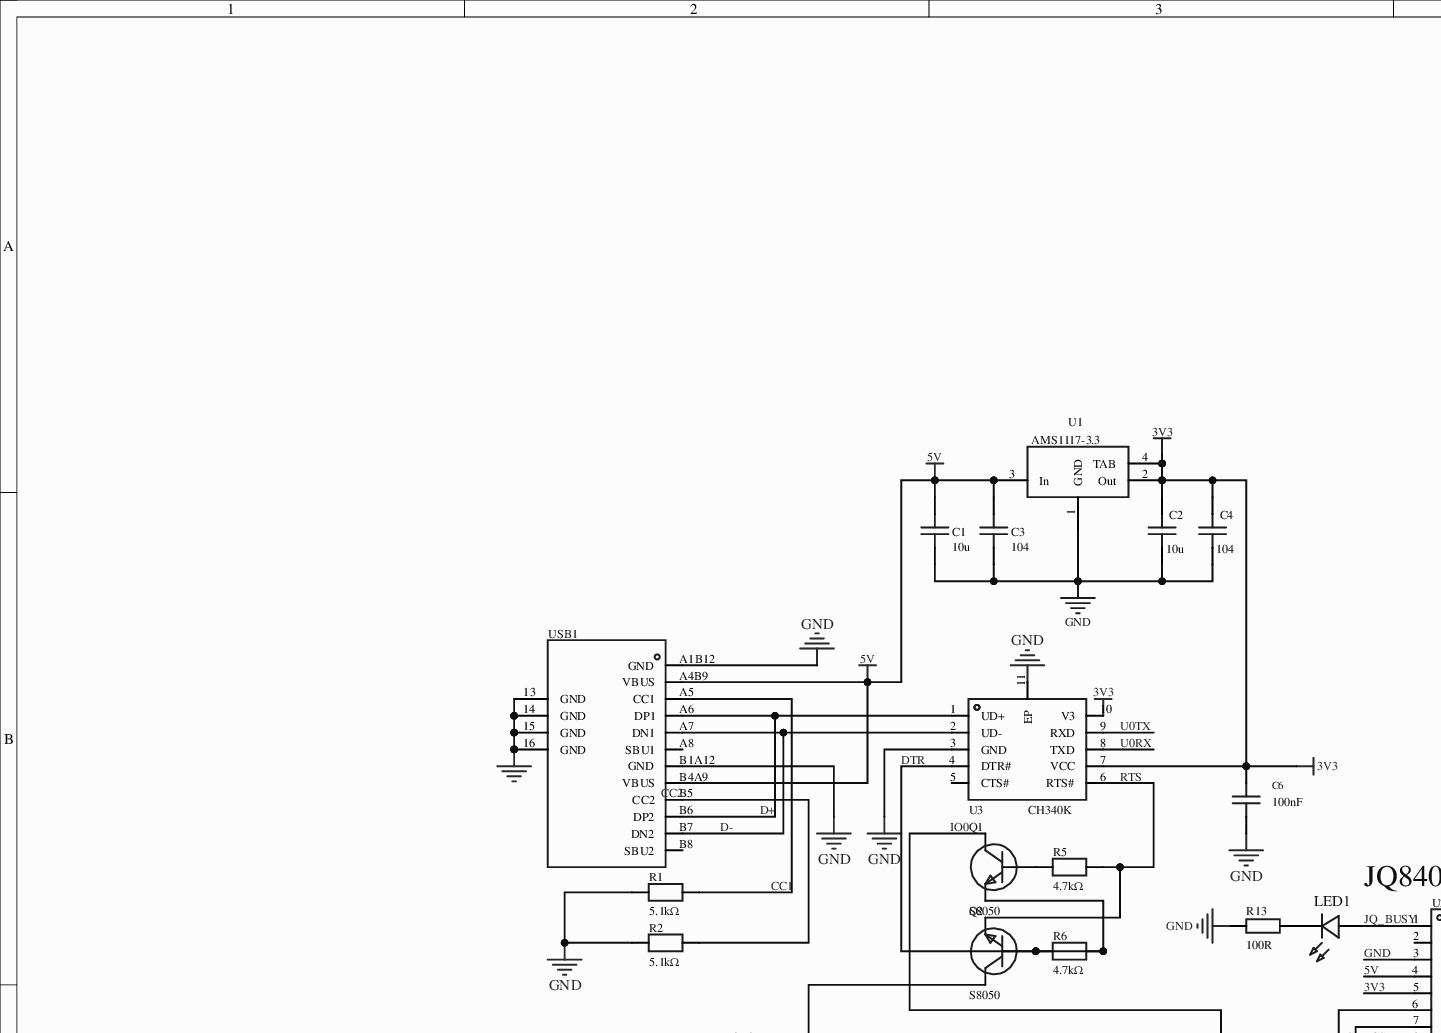
[diagram p0: MISC50923-3.schdoc, top left]
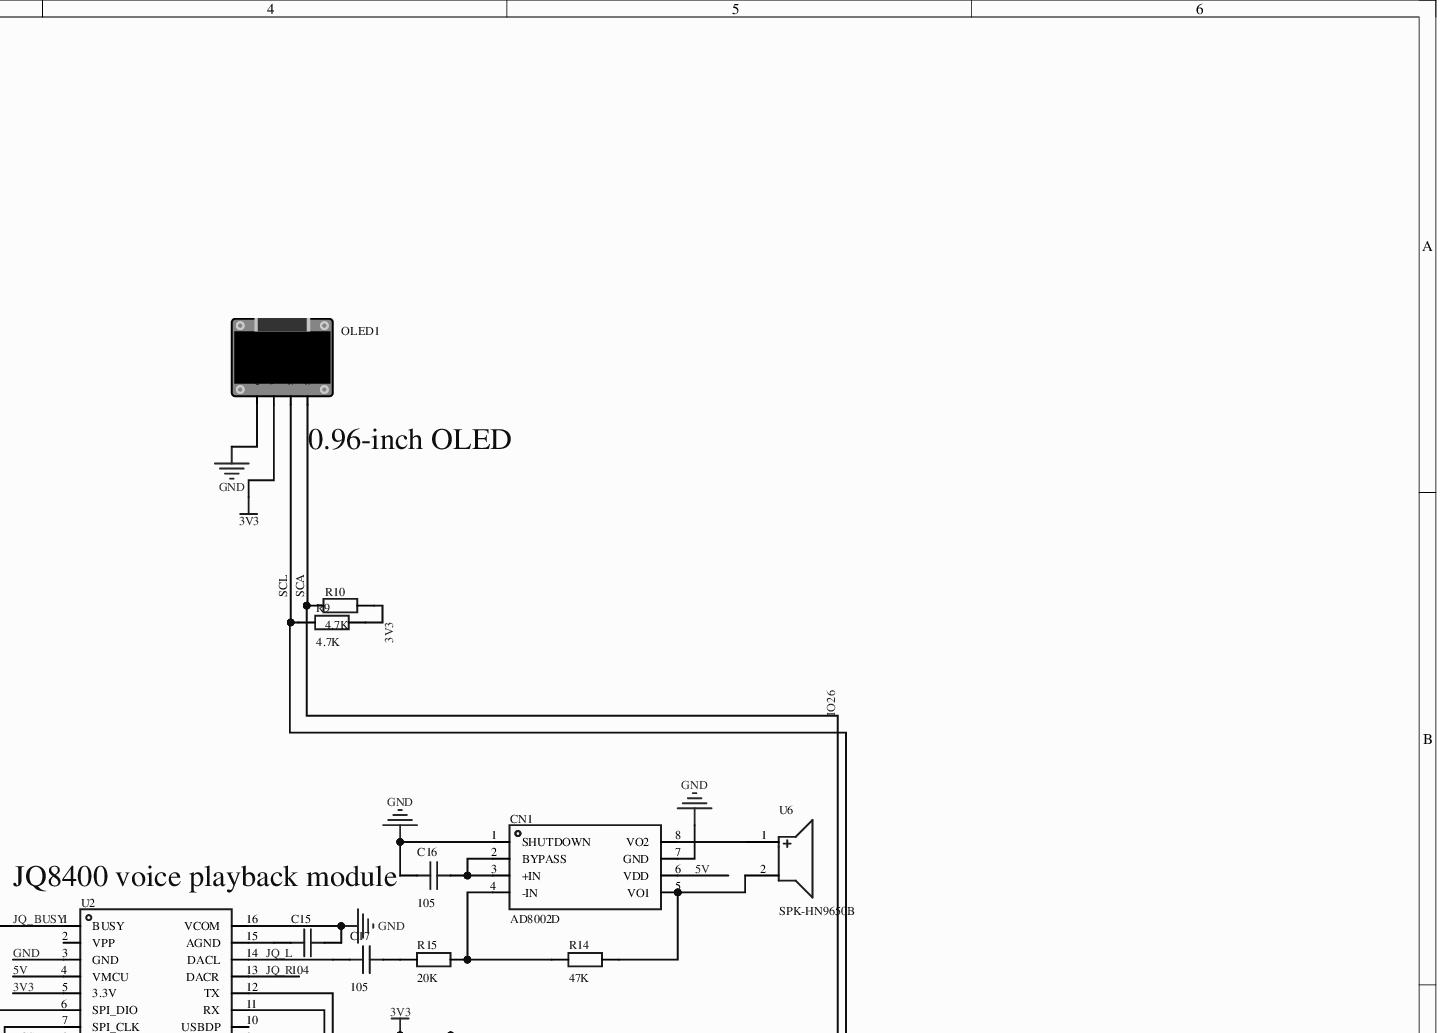
[diagram p1: MISC50923-3.schdoc, top right]
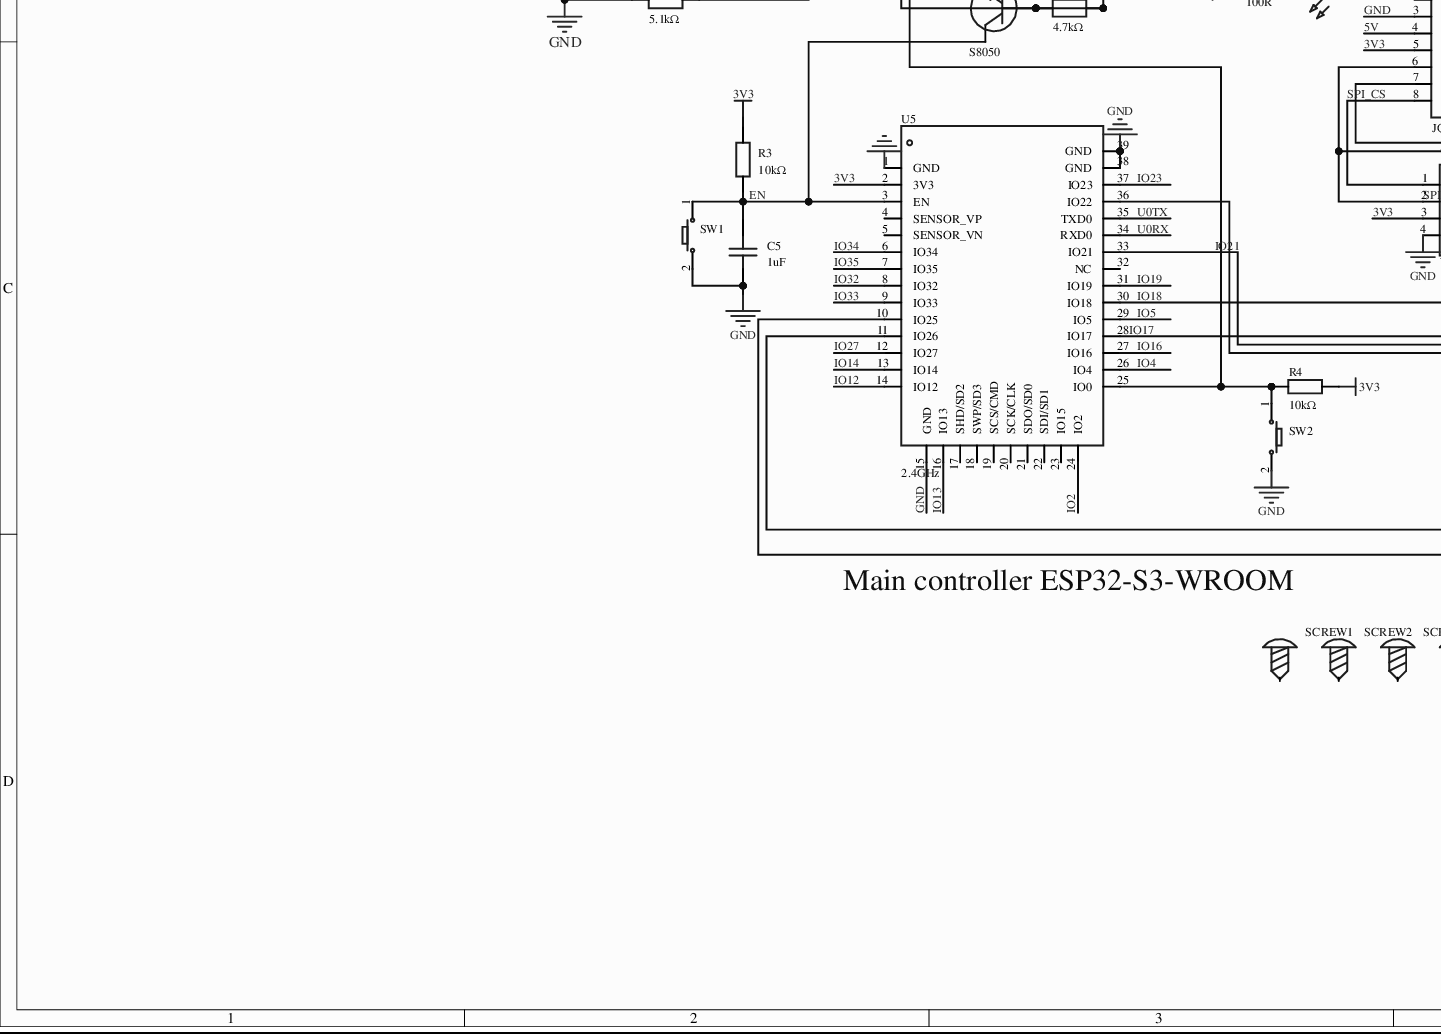
[diagram p2: MISC50923-3.schdoc, bottom left]
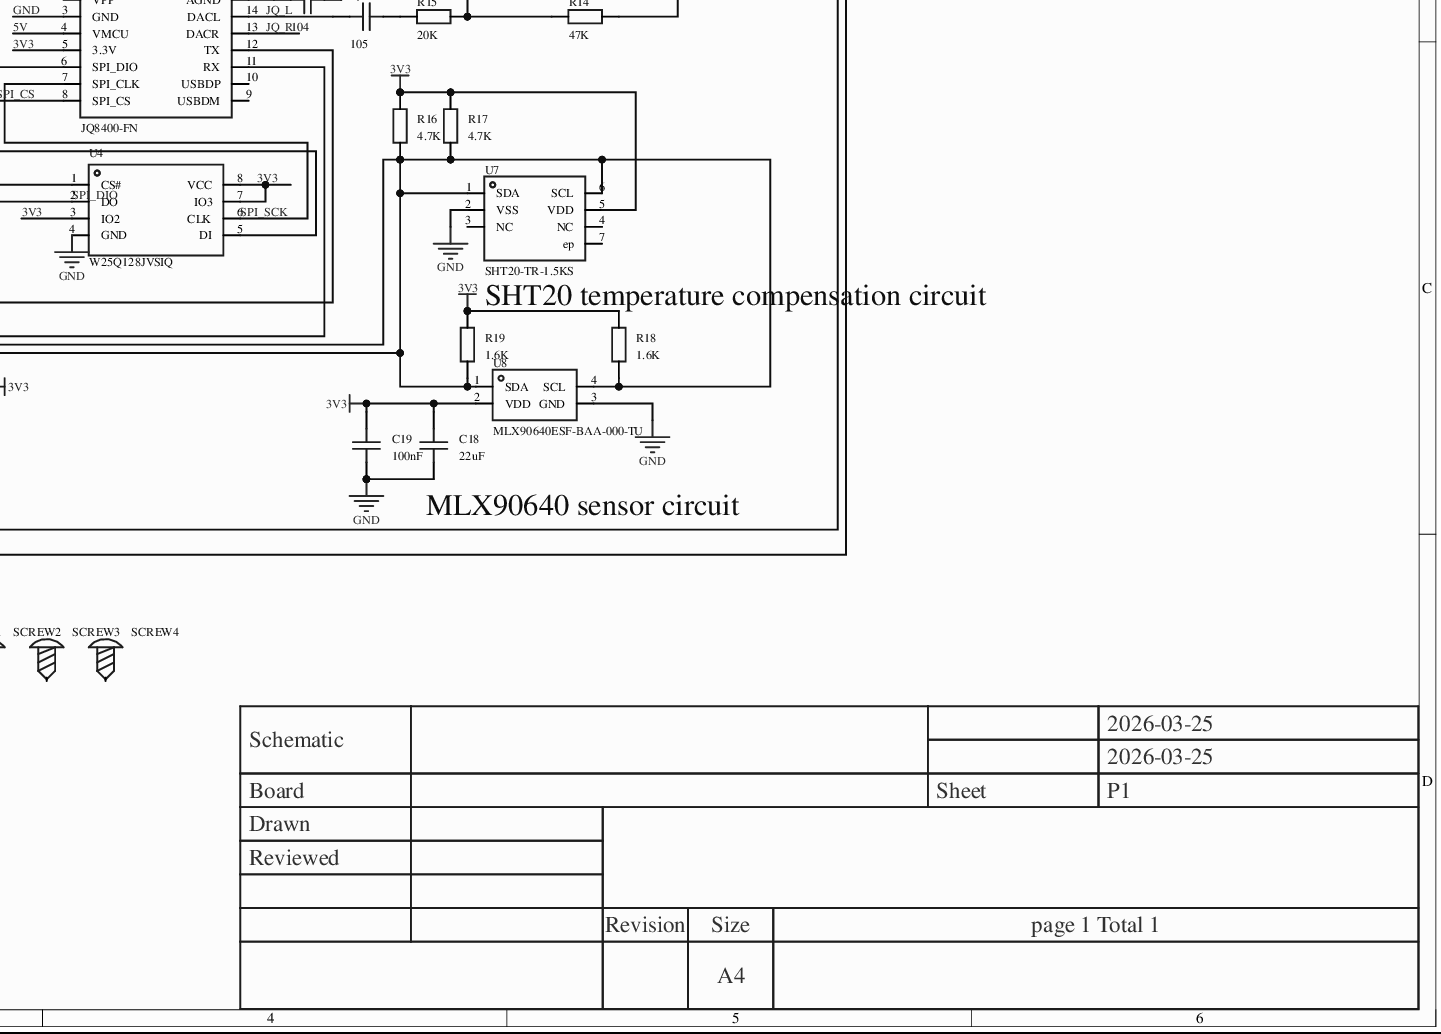
[diagram p3: MISC50923-3.schdoc, bottom right]
# Altium project MISC50923-2.PrjPcb
1 sheet, 46 parts. Net scope: global (net labels, ports and power ports of the same name join across sheets).
Board file: MISC50923.pcbdoc

## Sheet MISC50923-3.schdoc
size 420 x 297 mm; Version: V1.0; @Project Name: MISC50923; @Update Date: 2026-04-09; @Create Date: 2026-04-09; @Board Name: MISC50923; @Create Time: 11:05:08; @Page Count: 1; @Page No: 1; @Schematic Name: MISC50923; @Update Time: 11:05:08; Size: A4

### Parts
C1  10u  [C0805]
C2  10u  [C0805]
C3  104  [C0805]
C4  104  [C0805]
C5  1uF  [C0603]
C6  100nF  [C0603_1]
C15  104  [C0805]
C16  105  [C0805]
C17  105  [C0805]
C18  22uF  [C0805_1]
C19  100nF  [C0805_1]
CN1  AD8002D  [SOP-8_L5.0-W3.8-P1.27-LS6.0-BL]
LED1  (no value)  [LED_0603]
OLED1  (no value)  [0.96OLED_4P]
Q1  S8050  [SOT-23]
Q2  S8050  [SOT-23]
R1  5.1kΩ  [R0603]
R2  5.1kΩ  [R0603]
R3  10kΩ  [R0603]
R4  10kΩ  [R0603]
R5  4.7kΩ  [R0603]
R6  4.7kΩ  [R0603]
R9  4.7K  [R0805]
R10  4.7K  [R0805]
R13  100R  [R0603]
R14  47K  [R0603]
R15  20K  [R0603]
R16  4.7K  [R0603]
R17  4.7K  [R0603]
R18  1.6K  [R0603]
R19  1.6K  [R0603]
SCREW1  (no value)  [M3螺丝]
SCREW2  (no value)  [M3螺丝]
SCREW3  (no value)  [M3螺丝]
SCREW4  (no value)  [M3螺丝]
SW1  (no value)  [Key_SMD_3x4x2]
SW2  (no value)  [Key_SMD_3x4x2]
U1  AMS1117-3.3  [SOT-223_L6.5-W3.5-P2.30-LS7.0-BR]
U2  JQ8400-FN  [SOP-16_L9.9-W3.9-P1.27-LS6.0-BL]
U3  CH340K  [ESOP-10_L4.9-W3.9-P1.00-LS6.2-BL-EP]
U4  W25Q128JVSIQ  [SOIC-8_L5.3-W5.3-P1.27-LS8.0-BL]
U5  2.4GHz  [WIFIM-SMD_ESP32-WROOM-32-N4]
U6  SPK-HN9650B  [BUZ-SMD_L9.6-W9.6-LS10.0-R]
U7  SHT20-TR-1.5KS  [DFN-6_L3.0-W3.0-P0.95-TR-EP]
U8  MLX90640ESF-BAA-000-TU  [TO-39_4P-BD9.3_MLX90640ESF-BAA-000-TU_H5.7]
USB1  (no value)  [USB-C-SMD_TYPEC-304-BCP16]

### Nets
3V3: C2.2 C4.2 C6.2 C18.2 C19.2 OLED1.2(VCC) R3.2 R4.2 R9.1 R10.1 R16.2 R17.2 R18.2 R19.2 U1.2(Out) U1.4(TAB) U2.5(3.3V) U3.7(VCC) U3.10(V3) U4.3(IO2) U4.7(IO3) U4.8(VCC) U5.2(3V3) U7.5(VDD) U8.2(VDD)
5V: C1.2 C3.2 CN1.6(VDD) U1.3(In) U2.4(VMCU) USB1.A4B9(VBUS) USB1.B4A9(VBUS)
GND: C1.1 C2.1 C3.1 C4.1 C5.2 C6.1 C15.1 C16.2 C18.1 C19.1 CN1.1(SHUTDOWN) CN1.7(GND) OLED1.1(GND) R1.2 R2.2 R13.1 SW1.2 SW2.2 U1.1(GND) U2.3(GND) U2.16(VCOM) U3.3(GND) U3.11(EP) U4.4(GND) U5.1(GND) U5.15(GND) U5.38(GND) U5.39(GND) U7.2(VSS) U8.3(GND) USB1.13(GND) USB1.14(GND) USB1.15(GND) USB1.16(GND) USB1.A1B12(GND) USB1.B1A12(GND)
CC1: R1.1 USB1.A5(CC1)
CC2: R2.1 USB1.B5(CC2)
D+: U3.1(UD+) USB1.A6(DP1) USB1.B6(DP2)
D-: U3.2(UD-) USB1.A7(DN1) USB1.B7(DN2)
DTR: Q1.2(E) Q2.1(B) R6.1 R6.2 U3.4(DTR#)
EN: C5.1 Q2.3(C) R3.1 SW1.1 U5.3(EN)
IO0: Q1.3(C) R4.1 SW2.1 U5.25(IO0)
IO2: U5.24(IO2)
IO4: U5.26(IO4)
IO5: U5.29(IO5)
IO12: U5.14(IO12)
IO13: U5.16(IO13)
IO14: U5.13(IO14)
IO16: U5.27(IO16)
IO17: U2.11(RX) U5.28(IO17)
IO18: U2.12(TX) U5.30(IO18)
IO19: U5.31(IO19)
IO21: R16.1 R17.1 R18.1 R19.1 U5.33(IO21) U5.36(IO22) U7.1(SDA) U7.6(SCL) U8.1(SDA) U8.4(SCL)  [also labelled IO22]
IO23: U5.37(IO23)
IO26: OLED1.4(SDA) R10.2 U5.11(IO26)
IO27: U5.12(IO27)
IO32: U5.8(IO32)
IO33: U5.9(IO33)
IO34: U5.6(IO34)
IO35: U5.7(IO35)
JQ_BUSY: LED1.2(A) U2.1(BUSY)
JQ_L: C17.2 U2.14(DACL)
JQ_R: U2.13(DACR)
RTS: Q2.2(E) R5.1 U3.6(RTS#)
SPI_CS: U2.8(SPI_CS) U4.1(CS#)
SPI_DIO: U2.6(SPI_DIO) U4.2(DO) U4.5(DI)
SPI_SCK: U2.7(SPI_CLK) U4.6(CLK)
U0RX: U3.8(TXD) U5.34(RXD0)
U0TX: U3.9(RXD) U5.35(TXD0)
NetC15_2: C15.2 U2.15(AGND)
NetC16_1: C16.1 CN1.2(BYPASS) CN1.3(+IN)
NetC17_1: C17.1 R15.1
NetCN1_4: CN1.4(-IN) R14.1 R15.2
NetCN1_5: CN1.5(VO1) R14.2 U6.2
NetCN1_8: CN1.8(VO2) U6.1
NetLED1_1: LED1.1(C) R13.2
NetOLED1_3: OLED1.3(SCL) R9.2 U5.10(IO25)
NetQ1_1: Q1.1(B) R5.2

Not connected (* = marked no-connect by the designer): SCREW1 1; SCREW2 1; SCREW3 1; SCREW4 1; U2 2(VPP) 9(USBDM) 10(USBDP); U3 5(CTS#)*; U5 4(SENSOR_VP) 5(SENSOR_VN) 17(SHD/SD2) 18(SWP/SD3) 19(SCS/CMD) 20(SCK/CLK) 21(SDO/SD0) 22(SDI/SD1) 23(IO15) 32(NC); U7 3(NC) 4(NC) 7(ep); USB1 A8(SBU1)* B8(SBU2)*

### Notes on the sheet
- (near OLED1) 0.96-inch OLED
- SCL
- SCA
- (near C16) JQ8400 voice playback module
- SHT20 temperature compensation circuit
- (near C18) MLX90640 sensor circuit
- Main controller ESP32-S3-WROOM
- 2026-03-25
- Schematic
- Board
- Sheet
- P1
- Drawn
- Reviewed
- Revision
- Size
- A4
- page 1 Total 1

### Library data of the parts
C1 C2 = 10u: Add into BOM: yes; Capacitance: 1u; Device: 10u; Symbol: 10u; Convert to PCB: yes; Origin Footprint: C0805; Supplier: YUJING; FootprintName: C0805
C3 C4 C15-C17 = 104: Add into BOM: yes; Capacitance: 1u; Device: 104; Symbol: 104; Convert to PCB: yes; Origin Footprint: C0805; Supplier: YUJING; FootprintName: C0805
C5 = 104: Add into BOM: yes; Origin Footprint: C0805; Capacitance: 1u; Device: 104; Symbol: 104; Convert to PCB: yes; Supplier: YUJING; FootprintName: C0603
C6 = GRM155R71H104KE14D: Capacitance: 100nF; Tolerance: ±10%; Rated voltage: 50V; Dielectric (temperature coefficient): X7R;; Manufacturer: muRata(村田); 3D Model: 36a51122f27c49738f86b3bfa98863e0; 3D Model Transform: 39.37,19.685,0,0,0,0,0,0,0; AddInBom: yes; ModelName: C0402_L1.0-W0.5-H0.5; Device: GRM155R71H104KE14D; Symbol: GRM155R71H104KE14D; Value: 100nF; LCSC Part Name: 100nF ±10% 50V; Supplier Footprint: 0402; Datasheet: https://atta.szlcsc.com/upload/public/pdf/source/20180326/C77020_39BD49C951FF1AF0DB1F1FAC5AC1E401.pdf; Voltage Rated: 50V; Temperature Coefficient: X7R; Supplier: LCSC; Manufacturer Part: GRM155R71H104KE14D; Supplier Part: C77020; JLCPCB Part Class: Extended library; FootprintName: C0603_1; ConvertToPcb: yes
C18 C19 = CAP_0805: Symbol: CapAcitance_1; 3D Model: 1ba041120af144c991958decab20d241; 3D Model Transform: 78.74,51.181,0,0,0,0,0,0.0005,0; ConvertToPcb: yes; ModelName: C0805_L2.0-W1.3-H1.3; Device: CAP_0805; Supplier Footprint: 0805; FootprintName: C0805_1; AddInBom: yes
  C18: Value: 22uF
  C19: Value: 100nF
CN1 = AD8002D: 功放类型:AB类功放;扬声器通道数:单声道;输出功率:3Wx1@4Ω；2Wx1@4Ω;静态电流(Iq):-;; Manufacturer: IDCHIP(英锐芯); AddInBom: yes; Class: Class AB amplifier; Speaker Channels: Mono; Output Power: 3Wx1@4Ω;2Wx1@4Ω; Total Harmonic Distortion + Noise (THD+N): 1%; Number of Inputs: 1 differential input pair; Voltage - Supply: 2.2V~5.5V; ModelId: 823e4ad1ee284f09bfed9f55dae295e00819f05c4eef4c71ace90d822a990e87; ModelTransform: 196.85,236.22,0,0,0,0,0,0,0; Device: AD8002D; Symbol: AD8002D; FootprintName: SOP-8_L5.0-W3.8-P1.27-LS6.0-BL; LCSC Part Name: 3W单声道带关断模式音频功率放大器; SupplierPart: C395456; ManufacturerPart: AD8002D; Supplier Footprint: SOP-8; JLCPCB Part Class: Extended Part; Datasheet: https://item.szlcsc.com/datasheet/AD8002D/376120.html; Supplier: LCSC; ConvertToPcb: yes; Quiescent Current: -; Signal-to-Noise Ratio: -; Power Supply Rejection Ratio (PSRR): -; Efficiency: -; Features: Analog voltage gain; enable/shutdown function; Operating Temperature: -; ModelName: SOP-8_L5.0-W3.8-P1.27-LS6.0-BL
LED1 = LED_0603-R: Symbol: LED_R; Convert to PCB: yes; 3D Model: dd8257b0d61a4cd7b68939a056e080950819f05c4eef4c71ace90d822a990e87; 3D Model Transform: 58.72,29.4,22.03,0,0,0,0,0,0; ModelName: LED-0603_R; Device: LED_0603-R; Add into BOM: yes; Supplier Footprint: 0603; FootprintName: LED_0603
OLED1 = 0.96OLED模块_4P: Symbol: 0.96OLED module_4P; ConvertToPcb: yes; ModelId: 79c000fdb68d45a296c2e9bedf4f90550819f05c4eef4c71ace90d822a990e87; ModelTransform: 1393.69792,1318.895,0,0,0,0,0,-560.079,-137.795; Device: 0.96OLED module_4P; AddInBom: yes; FootprintName: 0.96OLED_4P; Supplier Footprint: 插件; ModelName: 0.96OLED_4P
Q1 Q2 = S8050: Manufacturer: CJ; AddInBom: yes; ModelId: dd91bed6c7114a8387ef499cf979050b; Device: S8050; Symbol: S8050; Supplier: LCSC; Manufacturer Part: S8050; image: C2146.jpg; Supplier Part: C2146; JLCPCB Part Class: Basic; Origin Footprint 2: SOT-23; FootprintName: SOT-23; ConvertToPcb: yes; ModelName: SOT-23
R1 R2 R5 R6 = TC0350B5101T5E: Resistor type: thin-film resistor; Resistance: 5.1kΩ; Tolerance: ±0.1%; Power: 166.667mW;; Manufacturer: UNI-ROYAL(厚声); 3D Model: fc143cca1e79419f9cd78b61e9279f08; 3D Model Transform: 31.8897,63.7794,0,90,0,0,0,0,0; Temperature Coefficient: ±50ppm/℃; Overload Voltage (Max): 75V; AddInBom: yes; Device: TC0350B5101T5E; Symbol: TC0350B5101T5E; LCSC Part Name: 5.1kΩ±0.1%166.667mW; Manufacturer Part: TC0350B5101T5E; Supplier Footprint: 0603; JLCPCB Part Class: Extended library; Datasheet: https://atta.szlcsc.com/upload/public/pdf/source/20190821/C415096_9FDBDDB676579191B9D59042FEBFA88B.pdf; Supplier: LCSC; Type: Thin-film resistor; Power(Watts): 166.667mW; Operating Temperature Range: -55℃~+155℃; FootprintName: R0603; ConvertToPcb: yes; ModelName: R0603
  R1 R2: Supplier Part: C415096; Value: 5.1kΩ
  R5 R6: Value: 4.7kΩ
R3 R4 = 0603WAF1002T5E: Resistor type: thick-film resistor; Resistance: 10kΩ; Tolerance: ±1%; Power: 100mW; Max working voltage: 75V; Temperature coefficient: ±100ppm/℃;; Manufacturer: UNI-ROYAL(厚声); 3D Model: fc143cca1e79419f9cd78b61e9279f08; 3D Model Transform: 31.8897,63.7794,0,90,0,0,0,0,0; AddInBom: yes; Device: 0603WAF1002T5E; Symbol: Resistor; LCSC Part Name: 厚膜电阻 10kΩ ±1% 100mW; Supplier Part: C25804; Manufacturer Part: 0603WAF1002T5E; JLCPCB Part Class: Basic Part; Datasheet: https://atta.szlcsc.com/upload/public/pdf/source/20200306/C422600_1E6D84923E4A46A82E41ADD87F860B5C.pdf; Supplier: LCSC; Type: Thick-film resistor; Power(Watts): 100mW; Overload Voltage (Max): 75V; Temperature Coefficient: ±100ppm/℃; Operating Temperature Range: -55℃~+155℃; Supplier Footprint: 0603; Value: 10kΩ; FootprintName: R0603; ConvertToPcb: yes; ModelName: R0603
R9 R10 = Res_0805: Symbol: Resistor_1; 3D Model: 37a81e68749a4138bd2dfa6897b24b85; 3D Model Transform: 78.74,51.181,0,0,0,0,0,-0.0005,0; ConvertToPcb: yes; ModelName: R0805_L2.0-W1.3-H0.6; Device: Res_0805; Value: 4.7K; Supplier Footprint: 0805; FootprintName: R0805; AddInBom: yes
R13-R19 = Res_0603: Symbol: Resistor; ConvertToPcb: yes; ModelId: fc143cca1e79419f9cd78b61e9279f080819f05c4eef4c71ace90d822a990e87; ModelTransform: 31.8897,63.7794,0,90,0,0,0,0,0; Device: Res_0603; FootprintName: R0603; AddInBom: yes; Supplier Footprint: 0603; ModelName: R0603
  R13: Value: 100R
  R14: Value: 47K
  R15: Value: 20K
  R16 R17: Value: 4.7K
  R18 R19: Value: 1.6K
SCREW1-SCREW4 = M3螺丝: Device: M3 screw; Symbol: Screw hole; ConvertToPcb: yes; FootprintName: M3 screw; AddInBom: yes; Supplier Footprint: 插件
SW1 SW2 = Key_SMD_3x4x2: Symbol: Tactile switch x2; 3D Model: 63599cce708d48afbce1b0db003544770819f05c4eef4c71ace90d822a990e87; 3D Model Transform: 196.85,114.17,79.13,0,0,0,0,0,0; ConvertToPcb: yes; ModelName: SW-SMD_L4.0-W2.9-H2-LS5.0; Device: Key_SMD_3x4x2; Supplier Footprint: SMD; FootprintName: Key_SMD_3x4x2; AddInBom: yes
U1 = AMS1117-3.3: Manufacturer: AMS; Add into BOM: yes; Device: AMS1117-3.3; Symbol: AMS1117-3.3; Convert to PCB: yes; Origin Footprint: SOT-223_L6.5-W3.5-P2.30-LS7.0-BR; Supplier: LCSC; Manufacturer Part: AMS1117-3.3; image: C6186.jpg; Supplier Part: C6186; JLCPCB Part Class: Basic; FootprintName: SOT-223_L6.5-W3.5-P2.30-LS7.0-BR
U2 = JQ8400-FN: AddInBom: yes; ModelId: ed96d47c1e844792b3e705d722a1a1fa0819f05c4eef4c71ace90d822a990e87; ModelTransform: 389.763,236.22,0,0,0,0,0,0,0; Device: JQ8400-FN; Symbol: JQ8400-FN; FootprintName: SOP-16_L9.9-W3.9-P1.27-LS6.0-BL; LCSC Part Name: JQ8400-FN; SupplierPart: C9900000891; ManufacturerPart: JQ8400-FN; Supplier Footprint: SOP-16; JLCPCB Part Class: Extended Part; Supplier: LCSC; ConvertToPcb: yes; ModelName: SOP-16_L9.9-W3.9-P1.27-LS6.0-BL
U3 = CH340K: Application function: -; Interface protocol: -;; Manufacturer: WCH(南京沁恒); 3D Model: 154218974c894ddbb70273feac157d69; 3D Model Transform: 192.913,242.1255,0,0,0,0,0,0,0; AddInBom: yes; ModelName: ESOP-10_L4.9-W3.9-H1.4-P1.00-LS6.2-BL-EP; Device: CH340K; Symbol: CH340K; LCSC Part Name: CH340K USB转串口芯片 CH340; Supplier Footprint: ESOP-10-EP-150mil; Datasheet: https://atta.szlcsc.com/upload/public/pdf/source/20200819/C84681_ADBED554CE321879DBD6B1D06488689C.pdf; Applications Function: -; Protocol: -; Supplier: LCSC; Supplier Part: C968586; Manufacturer Part: CH340K; JLCPCB Part Class: Extended library; FootprintName: ESOP-10_L4.9-W3.9-P1.00-LS6.2-BL-EP; ConvertToPcb: yes
U4 = W25Q128JVSIQ: Interface type: SPI; Storage capacity: 128Mbit; Clock frequency (fc): 133MHz;; Manufacturer: Winbond(华邦); Symbol: W25Q128JVSIQTR; AddInBom: yes; Voltage - Supply: 2.7V~3.6V; Standby Supply Current: 1uA; Program / Erase Cycles: 100000 cycles; Page Programming Time (Tpp): 3ms; Block Erase Time(tBE): 120ms@(32KB); Data Retention - TDR (Year): 20 years; ModelId: f83d990ad74f400caf5ac920b77715080819f05c4eef4c71ace90d822a990e87; ModelName: SOIC-8_L5.3-W5.3-H1.9-LS7.9-P1.27; ModelTransform: 208.661,311.25654,0,0,0,0,-0.0005,0.0005,0; Device: W25Q128JVSIQ; FootprintName: SOIC-8_L5.3-W5.3-P1.27-LS8.0-BL; LCSC Part Name: 编带 支持双路/四路SPI接口的3V、128Mbit 串行闪存; SupplierPart: C97521; ManufacturerPart: W25Q128JVSIQ; Supplier Footprint: SOIC-8-208mil; JLCPCB Part Class: Basic Part; Datasheet: https://item.szlcsc.com/datasheet/W25Q128JVSIQ/98729.html; Supplier: LCSC; ConvertToPcb: yes; Interface: SPI; Memory Size: 128Mbit; Clock Frequency: 133MHz; Operating Temperature: -40℃~+85℃
U5 = ESP32-WROOM-32 (16MB): 核心芯片:ESP32-D0WDQ6芯片;频率:2.4GHz;发射功率:20.5dBm;; Manufacturer: ESPRESSIF(乐鑫); Utilized IC / Part: ESP32-D0WDQ6 chip; AddInBom: yes; Interface Type: I2C; SDIO; UART; I2S; ModelId: 21a29bc006e94898b6cb1539a247a2980819f05c4eef4c71ace90d822a990e87; ModelTransform: 708.73866,1003.97437,0,0,0,0,0,147.362,0; Device: ESP32-WROOM-32 (16MB); Symbol: ESP32-WROOM-32 (16MB); FootprintName: WIFIM-SMD_ESP32-WROOM-32-N4; LCSC Part Name: 不带固件; SupplierPart: C6191506; ManufacturerPart: ESP32-WROOM-32 (16MB); Supplier Footprint: -; JLCPCB Part Class: Extended Part; Datasheet: https://item.szlcsc.com/datasheet/ESP32-WROOM-32%2520(16MB)/7136551.html; Supplier: LCSC; ConvertToPcb: yes; Value: 2.4GHz; Output Power: 20.5dBm; ModelName: WIFIM-SMD_ESP32-WROOM-32-N4
U6 = SPK-HN9650B: AddInBom: yes; ModelId: d9f071f9511e4f7795b1f85db80854800819f05c4eef4c71ace90d822a990e87; ModelName: BUZ-SMD_L9.6-W9.6-H5.0; ModelTransform: 393.7,377.952,0,0,0,0,0,0,0; Device: SPK-HN9650B; Symbol: SPK-HN9650B; FootprintName: BUZ-SMD_L9.6-W9.6-LS10.0-R; LCSC Part Name: SPK-HN9650B; SupplierPart: C9900001784; ManufacturerPart: SPK-HN9650B; Supplier Footprint: BUZ-SMD_L9.6-W9.6; JLCPCB Part Class: Extended Part; Supplier: LCSC; ConvertToPcb: yes
U7 = SHT20-TR-1.5KS: Interface type: I2C;; Manufacturer: Sensirion(瑞士盛思锐); Symbol: SHT20; AddInBom: yes; Voltage - Supply: 2.1V~3.6V; ModelId: 52f2b115daa640e29d29785a6ef4542a0819f05c4eef4c71ace90d822a990e87; ModelName: DFN-6_L3.0-W3.0-H1.0-P0.95; ModelTransform: 118.11,117.327,0,270,0,0,0,0,0; Device: SHT20-TR-1.5KS; FootprintName: DFN-6_L3.0-W3.0-P0.95-TR-EP; LCSC Part Name: 1-100706-01 SHT20-TR-1.5KS; SupplierPart: C53865; ManufacturerPart: SHT20-TR-1.5KS; Supplier Footprint: DFN-6-EP(3x3); JLCPCB Part Class: Extended Part; Datasheet: https://item.szlcsc.com/datasheet/SHT20-TR-1.5KS/54881.html; Supplier: LCSC; ConvertToPcb: yes; Interface: I2C
U8 = MLX90640ESF-BAA-000-TU_C17380659: 传感器类型:-;光学格式(inch):-;有源像素阵列:32Hx24V;像素大小:-;; Manufacturer: Melexis(比利时迈来芯); AddInBom: yes; ModelId: 3193193190874ecdba1bee0576d3e7930819f05c4eef4c71ace90d822a990e87; ModelTransform: 382.973,366.141,0,0,0,0,-9.055,0,-251.968; Device: MLX90640ESF-BAA-000-TU_C17380659; Symbol: MLX90640ESF-BAA-000-TU_C17380659; FootprintName: TO-39_4P-BD9.3_MLX90640ESF-BAA-000-TU_H5.7; LCSC Part Name: 32x24 IR阵列; SupplierPart: C17380659; ManufacturerPart: MLX90640ESF-BAA-000-TU; Supplier Footprint: TO-39; JLCPCB Part Class: Extended Part; Datasheet: https://item.szlcsc.com/datasheet/MLX90640ESF-BAA-000-TU/18509830.html; Supplier: LCSC; ConvertToPcb: yes; Sensor Type: -; Optical Format(inch): -; Active Pixel Array: 32Hx24V; Pixel Size: -; Operating Temperature: -40℃~+85℃; ModelName: TO-39_4P-BD9.3_MLX90640ESF-BAA-000-TU_H5.7
USB1 = typec-304-bcp16: 连接器类型:Type-C;标准:USB 3.1;公母:母座;触点数量:16.0;端口数量:1;安装方式:卧贴;额定电流 - 电源:3A;工作温度范围:-25~+85;焊接温度(最大值):260;; Manufacturer: XUNPU(讯普); Welding Temperature (Max): 260; 3D Model: bb1eabbfbdeb4e438a7034f2ad448367; 3D Model Transform: 352,305.1,0,0,0,0,0,-47.6,-39.4; Connector Type: Type-C; Gender: Female; Number of Contacts: 16.0; Number of Ports: 1; Mounting Sytle: Horizontal mount; Current Rating - Power (Max): 3A; AddInBom: yes; Device: typec-304-bcp16; Symbol: TYPEC-304-BCP16; Operating Temperature Range: -25~+85; LCSC Part Name: TYPEC-304-BCP16; Supplier Part: C720629; Manufacturer Part: TYPEC-304-BCP16; Supplier Footprint: SMD; JLCPCB Part Class: ExtendedPart; Datasheet: https://atta.szlcsc.com/upload/public/pdf/source/20211022/DACD6552F639E9483017DE6DC0E61150.pdf; Supplier: LCSC; Standard: USB3.1; FootprintName: USB-C-SMD_TYPEC-304-BCP16; ConvertToPcb: yes; ModelName: USB-C-SMD_TYPEC-304-BCP16